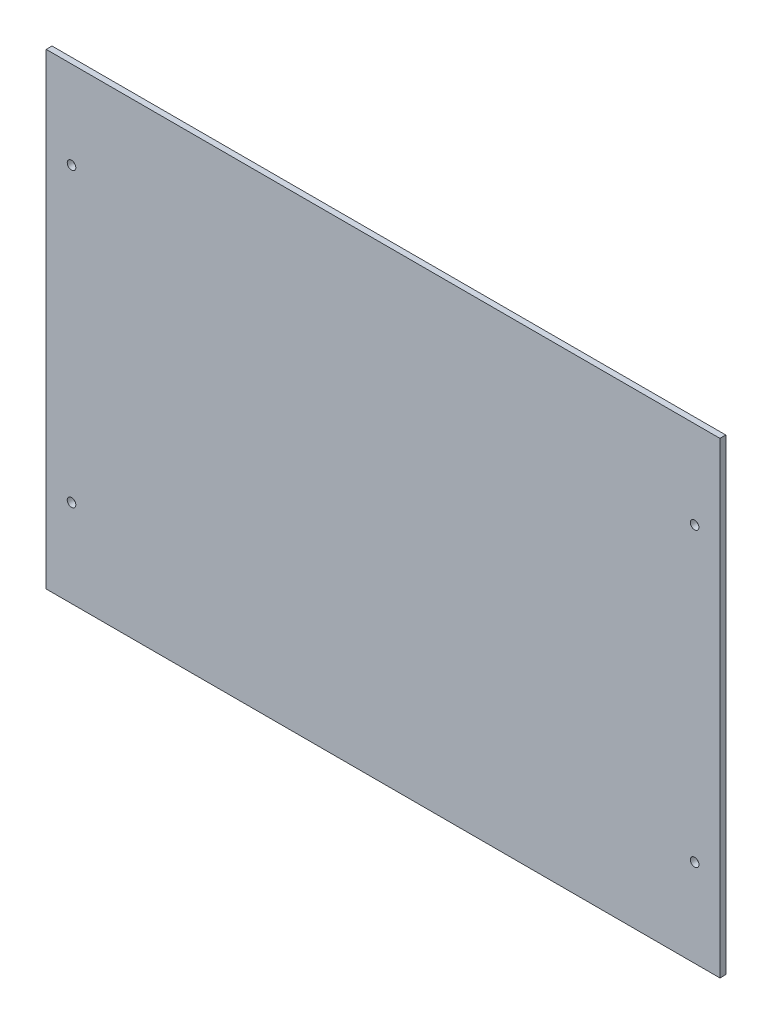
from build123d import *

# Parameters (mm, degrees)
SKETCH_1_W          = 346
SKETCH_1_H          = 240
EXTRUDE_1_DEPTH     = 3
SKETCH_2_R          = 2.2
CUT_EXTRUDE_1_DEPTH = 10


with BuildPart() as part:
    # 草图1 → 凸台-拉伸1 (new body)
    with BuildSketch(Plane.XY):
        Rectangle(SKETCH_1_W, SKETCH_1_H)
    extrude(amount=EXTRUDE_1_DEPTH)

    # 草图2 → 切除-拉伸1 (cut)
    with BuildSketch(Plane.XY.offset(3)):
        with Locations((160, 75)):
            Circle(SKETCH_2_R)
        with Locations((160, -75)):
            Circle(SKETCH_2_R)
        with Locations((-160, 75)):
            Circle(SKETCH_2_R)
        with Locations((-160, -75)):
            Circle(SKETCH_2_R)
        with Locations((-199.409999505, 140.432462879)):
            Circle(SKETCH_2_R)
        with Locations((-199.409999505, -9.567537121)):
            Circle(SKETCH_2_R)
    extrude(amount=-CUT_EXTRUDE_1_DEPTH, mode=Mode.SUBTRACT)


solid = part.part
